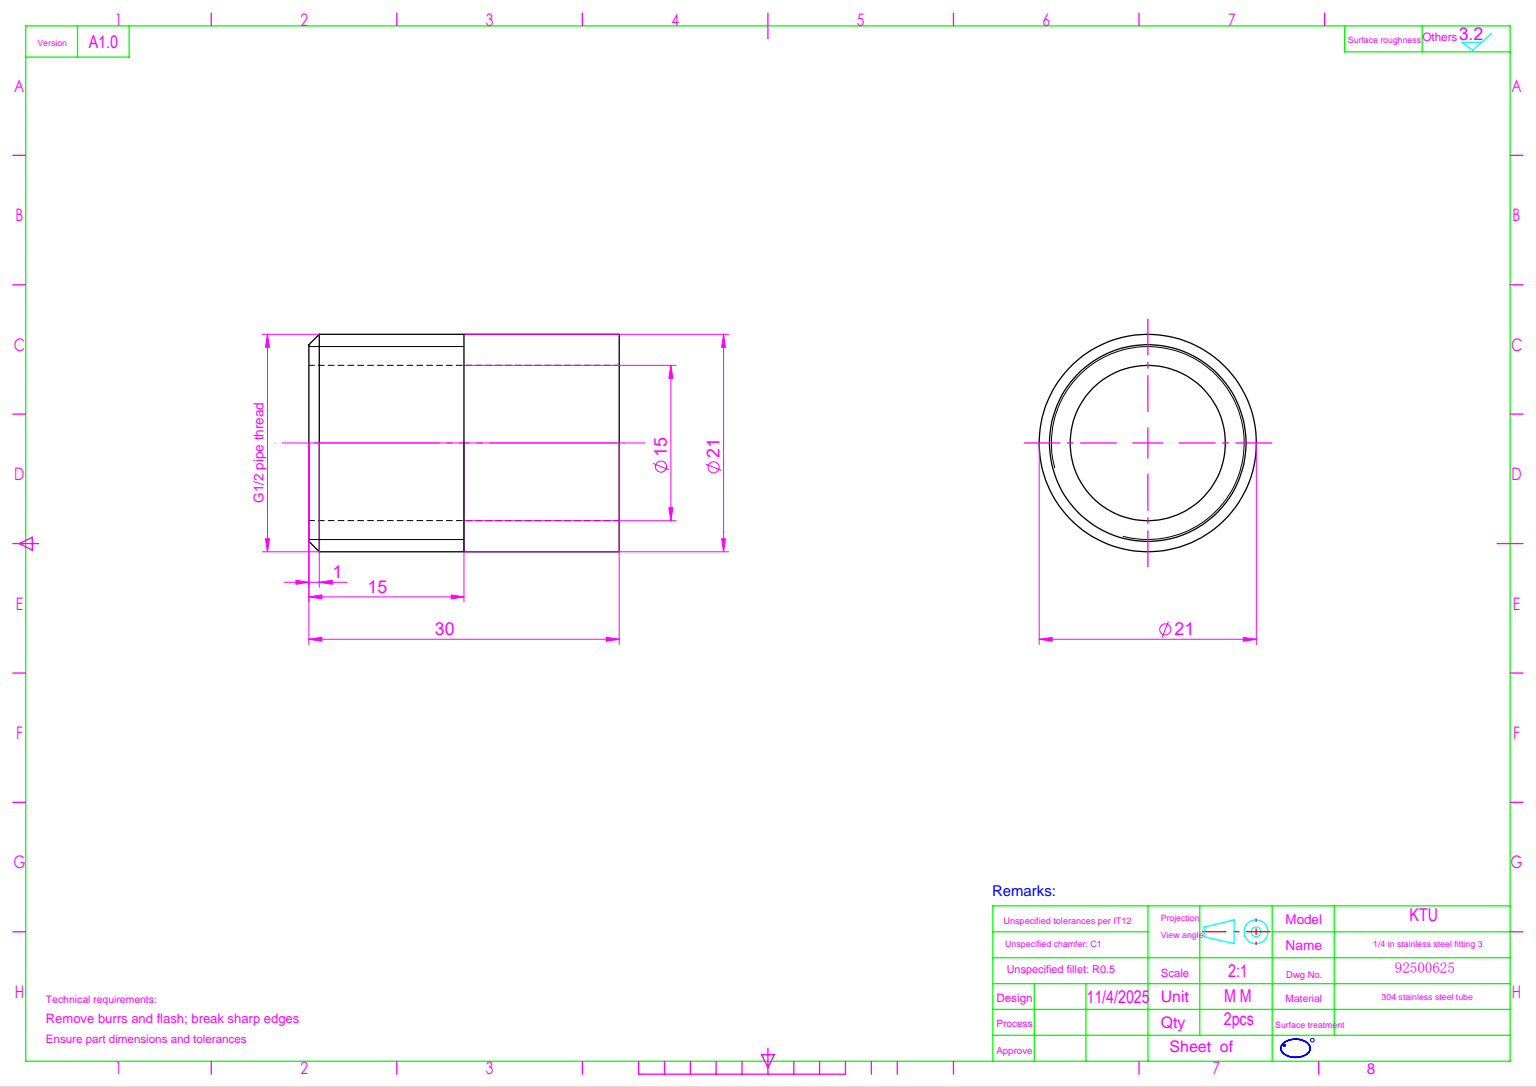
SolidWorks part; units mm, degrees
ref_plane "前视基准面" through (0, 0, 0) normal (0, 0, 1) x (1, 0, 0)
ref_plane "上视基准面" through (0, 0, 0) normal (0, 1, 0) x (1, 0, 0)
ref_plane "右视基准面" through (0, 0, 0) normal (1, 0, 0) x (0, 0, -1)
sketch "草图1" plane through (0, 0, 0) normal (1, 0, 0) x (0, 0, -1)
  circle A0 centre (0, 0) radius 10.5
  circle A1 centre (0, 0) radius 7.5
  dimension "D1" = 21
  dimension "D2" = 15
extrude "凸台-拉伸1" add sketch "草图1" along normal mid plane 30
cosmetic thread "装饰螺纹线1" parameters "D1"=15, "D2"=18.631
chamfer "倒角1" distance 1 angle 45 1 edges at (15, 0, -10.5)
